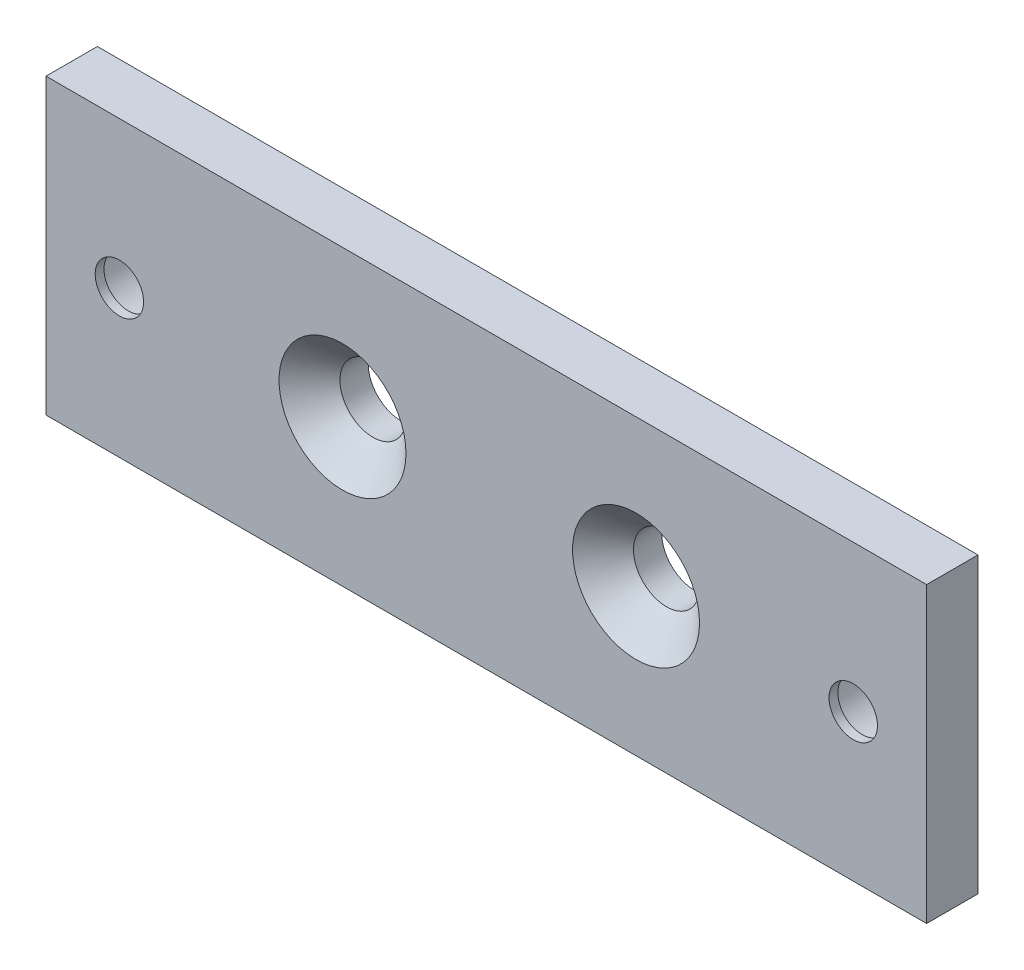
from build123d import *

# Parameters (mm, degrees)
SKETCH_1_W                  = 120
SKETCH_1_H                  = 40
EXTRUDE_1_DEPTH             = 4
HOLE_WIZARD_1_D             = 9
HOLE_WIZARD_1_DEPTH         = 10
HOLE_WIZARD_1_CSINK_D       = 17.3
HOLE_WIZARD_1_CSINK_ANGLE   = 90
HOLE_WIZARD_1_TIP           = 2.703872786
HOLE_WIZARD_1_2_D           = 6.6
HOLE_WIZARD_1_2_DEPTH       = 10
HOLE_WIZARD_1_2_CBORE_D     = 11
HOLE_WIZARD_1_2_CBORE_DEPTH = 6.8
HOLE_WIZARD_1_2_TIP         = 1.982840043
CHAMFER_1_SIZE              = 1


with BuildPart() as part:
    # 草图1 → 凸台-拉伸1 (new, symmetric)
    with BuildSketch(Plane.XY):
        Rectangle(SKETCH_1_W, SKETCH_1_H)
    extrude(amount=EXTRUDE_1_DEPTH, both=True)

    # Hole Wizard 1
    with Locations(Plane(origin=(-19.595917942, 0, 4), x_dir=(1, 0, 0), z_dir=(0, 0, 1))):
        with Locations((0, 0), (40, 0)):
            CounterSinkHole(HOLE_WIZARD_1_D / 2, HOLE_WIZARD_1_CSINK_D / 2, depth=HOLE_WIZARD_1_DEPTH, counter_sink_angle=HOLE_WIZARD_1_CSINK_ANGLE)
            with Locations((0, 0, -(HOLE_WIZARD_1_DEPTH + HOLE_WIZARD_1_TIP / 2))):  # 118° drill point
                Cone(0, HOLE_WIZARD_1_D / 2, HOLE_WIZARD_1_TIP, mode=Mode.SUBTRACT)

    # Hole Wizard 1 2
    with Locations(Plane(origin=(50, 0, -4), x_dir=(-1, 0, 0), z_dir=(0, 0, -1))):
        with Locations((0, 0), (100, 0)):
            CounterBoreHole(HOLE_WIZARD_1_2_D / 2, HOLE_WIZARD_1_2_CBORE_D / 2, HOLE_WIZARD_1_2_CBORE_DEPTH, depth=HOLE_WIZARD_1_2_DEPTH)
            with Locations((0, 0, -(HOLE_WIZARD_1_2_DEPTH + HOLE_WIZARD_1_2_TIP / 2))):  # 118° drill point
                Cone(0, HOLE_WIZARD_1_2_D / 2, HOLE_WIZARD_1_2_TIP, mode=Mode.SUBTRACT)

    # 倒角1
    chamfer_1_edges = [part.edges().sort_by_distance(p)[0] for p in [
        (0, -20, -4),
        (-60, 0, -4),
        (0, 20, -4),
        (60, 0, -4),
    ]]
    chamfer(chamfer_1_edges, length=CHAMFER_1_SIZE)


solid = part.part
